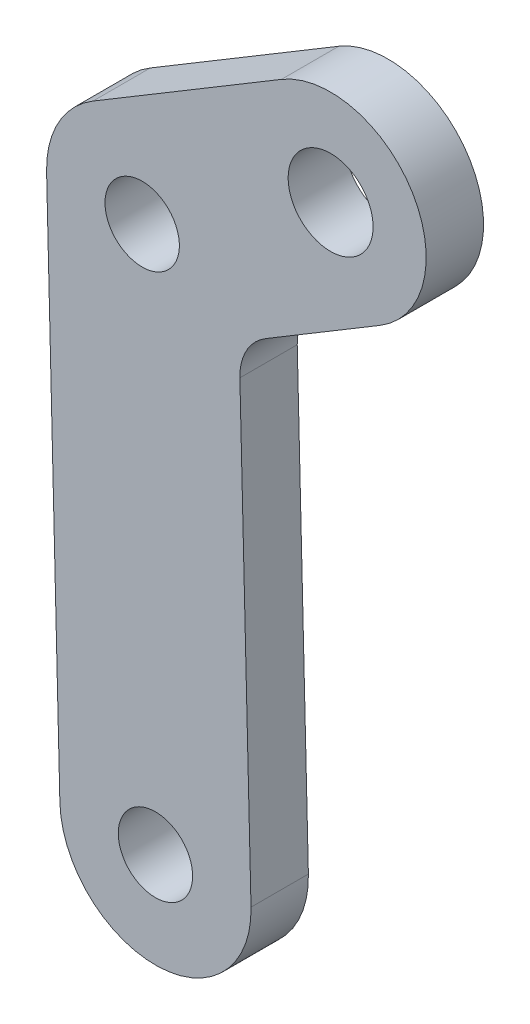
from build123d import *

# Parameters (mm, degrees)
SKETCH1_R           = 3.5
SKETCH1_R_2         = 4
BOSS_EXTRUDE1_DEPTH = 5.4


with BuildPart() as part:
    # Sketch1 → Boss-Extrude1 (new body)
    with BuildSketch(Plane.XY):
        with BuildLine():
            Line((-8.997274893, 37.552834761), (-7.747259547, -13.231665239))
            ThreePointArc((-7.747259547, -13.231665239), (1.471475273, -22.007480205), (10.247290239, -12.788745384))
            Line((10.247290239, -12.788745384), (9.197993195, 29.841151848))
            ThreePointArc((9.197993195, 29.841151848), (9.816337009, 32.376738458), (11.627190957, 34.256194898))
            Line((11.627190957, 34.256194898), (22.36781842, 40.697064727))
            ThreePointArc((22.36781842, 40.697064727), (25.457229961, 53.042113109), (13.11218158, 56.13152465))
            Line((13.11218158, 56.13152465), (-4.628608734, 45.492842556))
            ThreePointArc((-4.628608734, 45.492842556), (-7.885246166, 42.11283049), (-8.997274893, 37.552834761))
        make_face()
        with Locations(Location((0, 37.774294688, 0), (0, 0, 180))):
            Circle(SKETCH1_R, mode=Mode.SUBTRACT)
        with Locations(Location((1.250015346, -13.010205312, 0), (0, 0, 180))):
            Circle(SKETCH1_R, mode=Mode.SUBTRACT)
        with Locations(Location((17.74, 48.414294688, 0), (0, 0, 180))):
            Circle(SKETCH1_R_2, mode=Mode.SUBTRACT)
    extrude(amount=BOSS_EXTRUDE1_DEPTH)


solid = part.part
